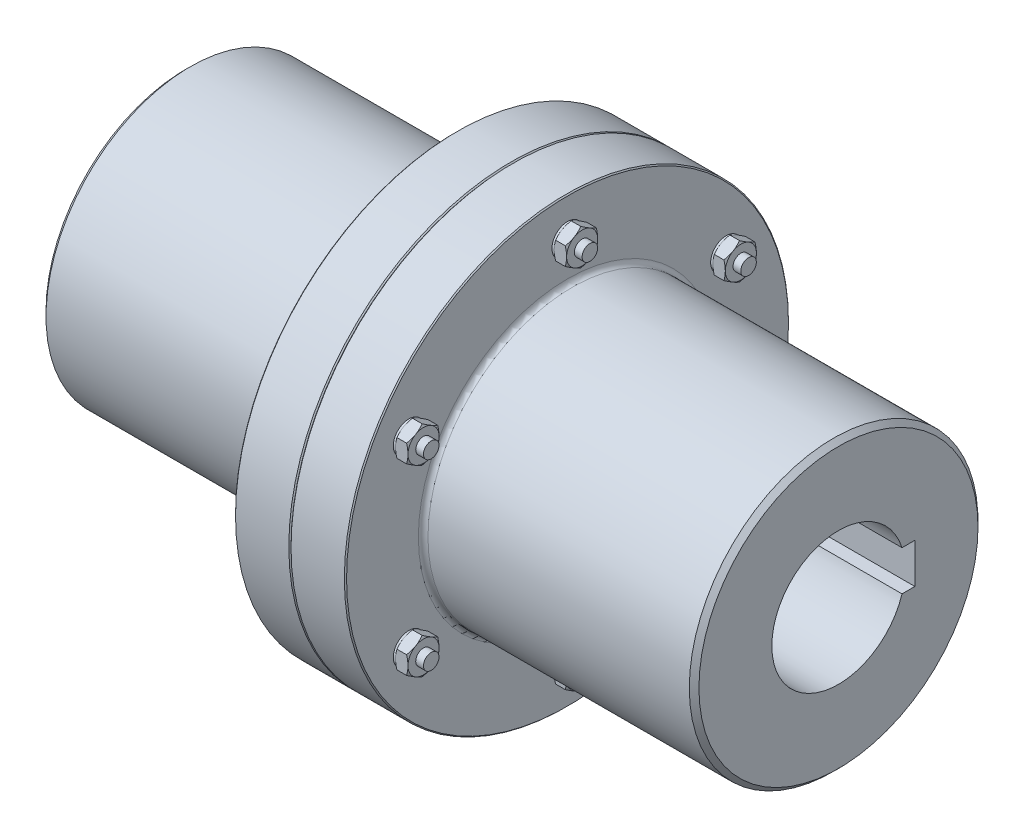
SolidWorks part; units mm, degrees
ref_plane "Front Plane" through (0, 0, 0) normal (0, 0, 1) x (1, 0, 0)
ref_plane "Top Plane" through (0, 0, 0) normal (0, 1, 0) x (1, 0, 0)
ref_plane "Right Plane" through (0, 0, 0) normal (1, 0, 0) x (0, 0, -1)
sketch "Sketch1" plane through (0, 0, 0) normal (0, 0, 1) x (1, 0, 0)
  line L0 (-147, 0) -> (147, 0) construction
  line L1 (0, 0) -> (0, 100) construction
  line L2 (25, 100) -> (-25, 100)
  line L3 (-25, 100) -> (-25, 65)
  line L4 (-25, 65) -> (-147, 65)
  line L5 (-147, 65) -> (-147, 0)
  line L6 (5, 70) -> (-5, 70)
  line L7 (-5, 70) -> (-5, 0)
  line L8 (-5, 37.5) -> (-147, 37.5)
  line L9 (-147, 38.5) -> (-146, 37.5)
  line L10 (-146, 37.5) -> (-146, 0)
  line L11 (-147, 2) -> (-5, 2)
  line L12 (25, 100) -> (25, 65)
  line L13 (147, 2) -> (5, 2)
  line L14 (146, 30) -> (146, 0)
  line L15 (147, 31) -> (146, 30)
  line L16 (5, 30) -> (147, 30)
  line L17 (5, 70) -> (5, 0)
  line L18 (147, 65) -> (147, 0)
  line L19 (25, 65) -> (147, 65)
  line L20 (-25, 82.5) -> (25, 82.5) construction
  line L21 (-25, 86) -> (25, 86)
  point P29 (0, 70)
  dimension "L" = 142
  dimension "S" = 10
  dimension "d1" = 75
  dimension "(D1)" = 130
  dimension "b" = 50
  dimension "D" = 200
  dimension "D22" = 165
  dimension "沉孔d1" = 140
  dimension "D4" = 1
  dimension "D5" = 45
  dimension "D6" = 4
  dimension "D7" = 1
  dimension "螺母d" = 7
  dimension "d2" = 60
  dimension "D8" = 45
  dimension "L2" = 142
sketch "Sketch14" plane through (0, 0, 0) normal (1, 0, 0) x (0, 0, -1)
  line L0 (0, 0) -> (-42.4, 0) construction
  line L1 (-42.4, 0) -> (-42.4, 10)
  line L2 (-42.4, 10) -> (-36.1421, 10)
  line L3 (0, 0) -> (0, 100) construction
  line L4 (0, 0) -> (0, 100) construction
  line L6 (42.4, 10) -> (36.1421, 10)
  line L7 (42.4, 0) -> (42.4, 10)
  line L8 (0, 0) -> (-21.2, -36.7195) construction
  line L9 (0, 0) -> (37.5, 0) construction
  line L10 (-21.2, -36.7195) -> (-29.8603, -31.7195)
  line L11 (-29.8603, -31.7195) -> (-26.7313, -26.3)
  line L12 (0, 0) -> (18.75, 32.476) construction
  circle A0 centre (0, 0) radius 37.5
  point P4 (-37.5, 0)
  point P12 (37.5, 0)
  dimension "D1" = 120
  dimension "b1" = 20
  dimension "t1" = 79.9
  dimension "B型t" = 79.9
  dimension "B型b" = 20
sketch "Sketch2" plane through (0, 0, 0) normal (0, 0, 1) x (1, 0, 0)
  line L0 (-147, 65) -> (-147, 0) construction
  line L1 (-25, 65) -> (-147, 65) construction
  line L2 (-25, 100) -> (-25, 65) construction
  line L3 (25, 100) -> (-25, 100) construction
  line L4 (0, 0) -> (0, 100) construction
  line L5 (5, 70) -> (-5, 70) construction
  line L6 (-5, 70) -> (-5, 0) construction
  line L8 (-147, 65) -> (-147, 0)
  line L9 (-25, 65) -> (-147, 65)
  line L10 (-25, 100) -> (-25, 65)
  line L11 (0, 100) -> (-25, 100)
  line L12 (0, 70) -> (0, 100)
  line L13 (0, 70) -> (-5, 70)
  line L14 (-5, 70) -> (-5, 0)
  line L15 (-147, 0) -> (-5, 0)
  line L18 (-147, 0) -> (147, 0) construction
  line L21 (-147, 0) -> (147, 0) construction
revolve "Revolve1" add sketch "Sketch2" angle 360 mid plane about L21
chamfer "Chamfer1" distance 2.1667 angle 45 1 edges at (-147, 0, 65)
chamfer "Chamfer2" distance 0.5 angle 45 2 edges at (0, 0, 100) (-25, 0, 100)
fillet "Fillet1" radius 1 1 edges at (-25, 0, 65)
sketch "Sketch15" plane through (0, 0, 0) normal (1, 0, 0) x (0, 0, -1)
  circle A0 centre (0, 0) radius 37.5 construction
  circle A1 centre (0, 0) radius 37.5
extrude "Cut-Extrude5" cut sketch "Sketch15" against normal through all
sketch "Sketch20" plane through (0, 0, 0) normal (1, 0, 0) x (0, 0, -1)
  line L0 (42.4, 10) -> (36.1421, 10) construction
  line L1 (42.4, 0) -> (42.4, 10) construction
  line L2 (0, 0) -> (37.5, 0) construction
  line L3 (42.4, 10) -> (36.1421, 10)
  line L4 (42.4, -10) -> (42.4, 10)
  line L5 (0, 0) -> (37.5, 0) construction
  line L6 (42.4, -10) -> (36.1421, -10)
  circle A0 centre (0, 0) radius 37.5 construction
  circle A1 centre (0, 0) radius 37.5
extrude "Cut-Extrude7" cut sketch "Sketch20" against normal through all contours A1 L6 L4 L3
sketch "Sketch22" [suppressed] plane through (0, 0, 0) normal (1, 0, 0) x (0, 0, -1)
  line L0 (0, 0) -> (-6.15, -10.6521) construction
  line L1 (-8.7481, -9.1521) -> (-7.105, -6.3062) construction
  line L2 (-6.15, -10.6521) -> (-8.7481, -9.1521) construction
  line L3 (0, 0) -> (-6.15, -10.6521) construction
  line L4 (-8.7481, -9.1521) -> (-7.105, -6.3062)
  line L5 (-3.5519, -12.1521) -> (-8.7481, -9.1521)
  line L6 (-3.5519, -12.1521) -> (-1.9089, -9.3062)
  circle A0 centre (0, 0) radius 9.5 construction
  circle A1 centre (0, 0) radius 9.5
extrude "Cut-Extrude8" [suppressed] cut sketch "Sketch22" against normal through all contours L3 A1 L4 L5 | A1 L3 L5 L6
sketch "Sketch23" [suppressed] plane through (0, 0, 0) normal (1, 0, 0) x (0, 0, -1)
  line L0 (-12.3, 3) -> (-9.0139, 3) construction
  line L1 (-12.3, 0) -> (-12.3, 3) construction
  line L2 (0, 0) -> (-12.3, 0) construction
  line L3 (-12.3, 3) -> (-9.0139, 3)
  line L4 (-12.3, -3) -> (-12.3, 3)
  line L5 (0, 0) -> (-12.3, 0) construction
  line L6 (-12.3, -3) -> (-9.0139, -3)
  circle A0 centre (0, 0) radius 9.5 construction
  circle A1 centre (0, 0) radius 9.5
extrude "Cut-Extrude9" [suppressed] cut sketch "Sketch23" against normal through all contours L5 A1 L3 L4 | A1 L5 L4 L6
sketch "Sketch3" plane through (0, 0, 0) normal (0, 0, 1) x (1, 0, 0)
  line L0 (25, 100) -> (-25, 100) construction
  line L1 (25, 100) -> (25, 65) construction
  line L2 (25, 65) -> (147, 65) construction
  line L3 (147, 65) -> (147, 0) construction
  line L4 (5, 70) -> (-5, 70) construction
  line L5 (5, 70) -> (5, 0) construction
  line L9 (25, 100) -> (0, 100)
  line L10 (25, 100) -> (25, 65)
  line L11 (25, 65) -> (147, 65)
  line L12 (147, 65) -> (147, 30)
  line L13 (5, 70) -> (0, 70)
  line L14 (5, 70) -> (5, 0)
  line L15 (5, 0) -> (147, 0)
  line L16 (-147, 0) -> (147, 0) construction
  line L17 (147, 30) -> (147, 0)
  line L18 (0, 100) -> (0, 70)
  line L19 (-147, 0) -> (147, 0) construction
revolve "Revolve2" add sketch "Sketch3" angle 360 mid plane about L19
sketch "Sketch16" plane through (0, 0, 0) normal (1, 0, 0) x (0, 0, -1)
  line L0 (0, 0) -> (-17.2, -29.7913) construction
  line L1 (0, 0) -> (-100, 0) construction
  line L2 (-34.4, -9) -> (-34.4, 9) construction
  line L3 (-34.4, 9) -> (-28.6182, 9) construction
  line L4 (-34.4, -9) -> (-28.6182, -9) construction
  line L5 (0, 0) -> (0, 100) construction
  line L6 (0, 0) -> (0, 100) construction
  line L7 (34.4, -9) -> (28.6182, -9) construction
  line L8 (34.4, 9) -> (28.6182, 9) construction
  line L9 (34.4, -9) -> (34.4, 9) construction
  line L10 (0, 0) -> (34.4, 0) construction
  line L12 (-9.4058, -34.2913) -> (-24.9942, -25.2913) construction
  line L13 (-24.9942, -25.2913) -> (-22.1033, -20.2841) construction
  line L14 (-9.4058, -34.2913) -> (-6.5149, -29.2841) construction
  line L15 (0, 0) -> (15, 25.9808) construction
  circle A0 centre (0, 0) radius 30
  circle A1 centre (0, 0) radius 100 construction
  point P7 (-30, 0)
  point P12 (-34.4, 0)
  point P19 (34.4, 0)
  point P20 (30, 0)
  dimension "D1" = 120
  dimension "b2" = 18
  dimension "t2" = 64.4
  dimension "D2" = 18
  dimension "D3" = 64.4
extrude "Cut-Extrude6" cut sketch "Sketch16" along normal through all
sketch "Sketch24" plane through (0, 0, 0) normal (1, 0, 0) x (0, 0, -1)
  line L6 (34.4, 9) -> (28.6182, 9) construction
  line L7 (34.4, -9) -> (34.4, 9) construction
  line L8 (34.4, -9) -> (28.6182, -9) construction
  line L9 (34.4, 9) -> (28.6182, 9)
  line L10 (34.4, -9) -> (34.4, 9)
  line L11 (34.4, -9) -> (28.6182, -9)
  circle A0 centre (0, 0) radius 30 construction
  circle A1 centre (0, 0) radius 30
extrude "Cut-Extrude10" cut sketch "Sketch24" along normal through all
sketch "Sketch25" [suppressed] plane through (0, 0, 0) normal (1, 0, 0) x (0, 0, -1)
  line L0 (-8.7481, -9.1521) -> (-7.105, -6.3062) construction
  line L1 (-3.5519, -12.1521) -> (-8.7481, -9.1521) construction
  line L2 (-3.5519, -12.1521) -> (-1.9089, -9.3062) construction
  line L3 (-8.7481, -9.1521) -> (-7.105, -6.3062)
  line L4 (-3.5519, -12.1521) -> (-8.7481, -9.1521)
  line L5 (-3.5519, -12.1521) -> (-1.9089, -9.3062)
  circle A0 centre (0, 0) radius 9.5 construction
  circle A1 centre (0, 0) radius 9.5
extrude "Cut-Extrude11" [suppressed] cut sketch "Sketch25" along normal through all contours A1 L3 L4 L5
sketch "Sketch26" [suppressed] plane through (0, 0, 0) normal (1, 0, 0) x (0, 0, -1)
  line L6 (-12.3, 3) -> (-9.0139, 3) construction
  line L7 (-12.3, -3) -> (-12.3, 3) construction
  line L8 (-12.3, -3) -> (-9.0139, -3) construction
  line L9 (-12.3, 3) -> (-9.0139, 3)
  line L10 (-12.3, -3) -> (-12.3, 3)
  line L11 (-12.3, -3) -> (-9.0139, -3)
  circle A0 centre (0, 0) radius 9.5 construction
  circle A1 centre (0, 0) radius 9.5
extrude "Cut-Extrude12" [suppressed] cut sketch "Sketch26" along normal through all
chamfer "Chamfer3" distance 0.5 angle 45 2 edges at (25, 0, 100) (0, 0, 100)
chamfer "Chamfer4" distance 2.1667 angle 45 1 edges at (147, 0, 65)
fillet "Fillet2" radius 2.1667 1 edges at (25, 0, 65)
sketch "Sketch6" plane through (-25, 0, 0) normal (-1, 0, 0) x (0, 0, 1)
  circle A0 centre (0, 82.5) radius 3.5
extrude "Cut-Extrude1" cut sketch "Sketch6" against normal up to vertex (50 mm away) up to point (25, 100, 0)
chamfer "Chamfer5" distance 0.2 angle 45 1 edges at (-25, 82.5, 3.5)
chamfer "Chamfer6" distance 0.2 angle 45 1 edges at (25, 82.5, 3.5)
pattern_circular "CirPattern1" count 6 over 360 about axis through (0, 0, 0) along (1, 0, 0) of "Cut-Extrude1", "Chamfer5", "Chamfer6"
sketch "Sketch7" plane through (0, 0, 0) normal (0, 0, 1) x (1, 0, 0)
  line L0 (-25, 82.5) -> (-25, 86)
  line L1 (-25, 86) -> (35.08, 86)
  line L2 (35.08, 86) -> (35.08, 82.5)
  line L3 (35.08, 82.5) -> (-25, 82.5)
  line L4 (-25, 100) -> (-25, 65) construction
  dimension "D1" = 60.08
revolve "Revolve3" add sketch "Sketch7" angle 360 mid plane about L3
sketch "Sketch8" plane through (-25, 0, 0) normal (-1, 0, 0) x (0, 0, 1)
  line L1 (0, 90.5829) -> (-7, 86.5415)
  line L2 (-7, 86.5415) -> (-7, 78.4585)
  line L3 (-7, 78.4585) -> (0, 74.4171)
  line L4 (0, 74.4171) -> (7, 78.4585)
  line L5 (7, 78.4585) -> (7, 86.5415)
  line L6 (7, 86.5415) -> (0, 90.5829)
  circle A0 centre (0, 82.5) radius 7 construction
  dimension "D1" = 14
extrude "Boss-Extrude1" add sketch "Sketch8" along normal blind 5.6
sketch "Sketch9" plane through (-30.6, 0, 0) normal (-1, 0, 0) x (0, 0, 1)
  circle A0 centre (0, 82.5) radius 7 construction
  circle A1 centre (0, 82.5) radius 7
  circle A2 centre (0, 82.5) radius 10.5
  dimension "D1" = 21
extrude "Cut-Extrude2" cut sketch "Sketch9" against normal blind 1 draft 60
sketch "Sketch10" plane through (25, 0, 0) normal (1, 0, 0) x (0, 0, -1)
  circle A0 centre (0, 82.5) radius 7
  dimension "D1" = 14
extrude "Boss-Extrude2" add sketch "Sketch10" along normal blind 1
sketch "Sketch11" plane through (26, 0, 0) normal (1, 0, 0) x (0, 0, -1)
  line L6 (7, 86.5415) -> (0, 90.5829)
  line L7 (7, 78.4585) -> (7, 86.5415)
  line L8 (0, 74.4171) -> (7, 78.4585)
  line L9 (-7, 78.4585) -> (0, 74.4171)
  line L10 (-7, 86.5415) -> (-7, 78.4585)
  line L11 (0, 90.5829) -> (-7, 86.5415)
  line L12 (7, 86.5415) -> (0, 90.5829)
  line L13 (7, 78.4585) -> (7, 86.5415)
  line L14 (0, 74.4171) -> (7, 78.4585)
  line L15 (-7, 78.4585) -> (0, 74.4171)
  line L16 (-7, 86.5415) -> (-7, 78.4585)
  line L17 (0, 90.5829) -> (-7, 86.5415)
  dimension "D1" = 0
extrude "Boss-Extrude3" add sketch "Sketch11" along normal blind 5.6
sketch "Sketch12" plane through (31.6, 0, 0) normal (1, 0, 0) x (0, 0, -1)
  circle A1 centre (0, 82.5) radius 10.5
  circle A2 centre (0, 82.5) radius 10.5
  circle A3 centre (0, 82.5) radius 7
  circle A4 centre (0, 82.5) radius 7
  dimension "D1" = 0
  dimension "D2" = 0
extrude "Cut-Extrude3" cut sketch "Sketch12" against normal blind 1 draft 60
sketch "Sketch13" plane through (26, 0, 0) normal (-1, 0, 0) x (0, 0, 1)
  circle A1 centre (0, 82.5) radius 7
  circle A2 centre (0, 82.5) radius 7
  circle A3 centre (0, 82.5) radius 10.5
  circle A4 centre (0, 82.5) radius 10.5
  dimension "D1" = 0
  dimension "D2" = 0
extrude "Cut-Extrude4" cut sketch "Sketch13" against normal blind 1 draft 60
pattern_circular "CirPattern3" count 6 over 360 about axis through (0, 0, 0) along (1, 0, 0) of "Revolve3", "Boss-Extrude1", "Cut-Extrude2", "Boss-Extrude2", "Boss-Extrude3", "Cut-Extrude3", "Cut-Extrude4"
